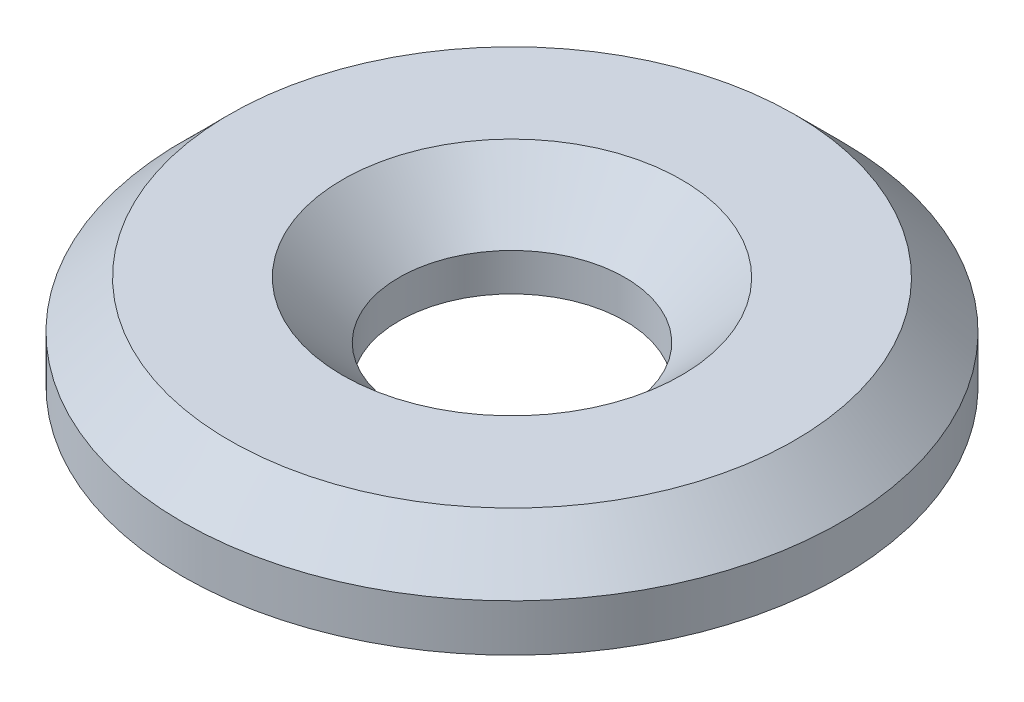
SolidWorks part; units mm, degrees
material "Commercially Pure titanium (Ti-55)  UNS R50550*"
ref_plane "Front Plane" through (0, 0, 0) normal (0, 0, 1) x (1, 0, 0)
ref_plane "Top Plane" through (0, 0, 0) normal (0, 1, 0) x (1, 0, 0)
ref_plane "Right Plane" through (0, 0, 0) normal (1, 0, 0) x (0, 0, -1)
sketch "Sketch1" plane through (0, 0, 0) normal (0, 0, 1) x (1, 0, 0)
  line L0 (0, 7.0385) -> (0, -7.0385) construction
  line L1 (9, 7.0385) -> (17.5, 7.0385)
  line L2 (17.5, 7.0385) -> (17.5, 2.0385)
  line L3 (17.5, 2.0385) -> (6, 2.0385)
  line L4 (6, 2.0385) -> (6, 4.0385)
  line L5 (6, 4.0385) -> (9, 7.0385)
  dimension "D1" = 35
  dimension "D2" = 2
  dimension "D3" = 5
  dimension "D4" = 45
  dimension "D5" = 12
revolve "Revolve1" add sketch "Sketch1" angle 360 about L0
chamfer "Chamfer1" distance 2.5 angle 45 1 edges at (0, 7.0385, 17.5)
